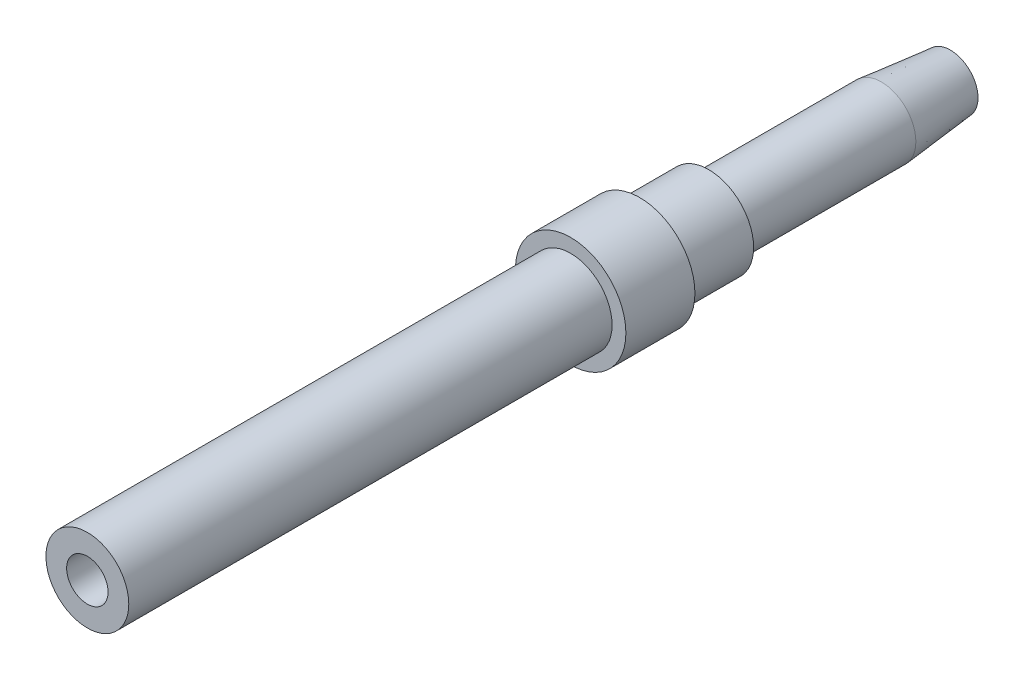
from build123d import *

# Parameters (mm, degrees)
SKETCH1_R           = 5
SKETCH1_R_2         = 3
BOSS_EXTRUDE1_DEPTH = 35
SKETCH2_R           = 6.5
SKETCH2_R_2         = 3
BOSS_EXTRUDE2_DEPTH = 10
SKETCH3_R           = 8
SKETCH3_R_2         = 3
BOSS_EXTRUDE3_DEPTH = 10
SKETCH4_R           = 6
SKETCH4_R_2         = 3
BOSS_EXTRUDE4_DEPTH = 70
CHAMFER1_SIZE       = 1
CHAMFER1_SIZE2      = 10


with BuildPart() as part:
    # Sketch1 → Boss-Extrude1 (new body)
    with BuildSketch(Plane.XY):
        Circle(SKETCH1_R)
        Circle(SKETCH1_R_2, mode=Mode.SUBTRACT)
    extrude(amount=BOSS_EXTRUDE1_DEPTH)

    # Sketch2 → Boss-Extrude2 (add)
    with BuildSketch(Plane.XY.offset(35)):
        Circle(SKETCH2_R)
        Circle(SKETCH2_R_2, mode=Mode.SUBTRACT)
    extrude(amount=BOSS_EXTRUDE2_DEPTH)

    # Sketch3 → Boss-Extrude3 (add)
    with BuildSketch(Plane.XY.offset(45)):
        Circle(SKETCH3_R)
        Circle(SKETCH3_R_2, mode=Mode.SUBTRACT)
    extrude(amount=BOSS_EXTRUDE3_DEPTH)

    # Sketch4 → Boss-Extrude4 (add)
    with BuildSketch(Plane.XY.offset(55)):
        Circle(SKETCH4_R)
        Circle(SKETCH4_R_2, mode=Mode.SUBTRACT)
    extrude(amount=BOSS_EXTRUDE4_DEPTH)

    # Chamfer1
    chamfer1_edges = [part.edges().sort_by_distance(p)[0] for p in [
        (-5, 0, 0),
    ]]
    chamfer1_side = [part.faces().sort_by_distance(p)[0] for p in [
        (-4.858578644, 0, 0),
    ]]
    chamfer(chamfer1_edges, length=CHAMFER1_SIZE, length2=CHAMFER1_SIZE2, reference=chamfer1_side[0])


solid = part.part
